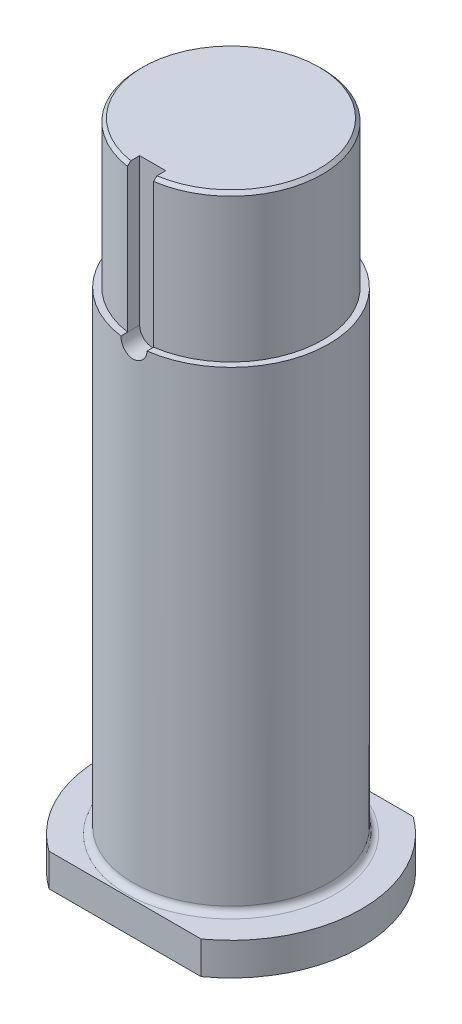
from build123d import *

# Parameters (mm, degrees)
SKETCH2_OUTSIDE_W   = 127.956
SKETCH2_OUTSIDE_H   = 127.956
SKETCH2_OUTSIDE_W_2 = 130
SKETCH2_OUTSIDE_H_2 = 65
CUT_EXTRUDE1_DEPTH  = 10
CUT_EXTRUDE2_REACH  = 213.642
CHAMFER1_SIZE       = 1
FILLET2_R           = 2


with BuildPart() as part:
    # Sketch1 → Revolve1 (revolve)
    with BuildSketch(Plane.XY, mode=Mode.PRIVATE) as revolve1_sk:
        Polygon((0, 0), (40, 0), (40, 10), (30, 10), (30, 155), (28, 155), (28, 200), (0, 200), align=None)
    revolve(revolve1_sk.sketch.rotate(Axis((0, 0, 0), (0, -1, 0)), 90), axis=Axis((0, 0, 0), (0, -1, 0)))

    # Sketch2 outside → Cut-Extrude1 (cut)
    with BuildSketch(Plane(origin=(0, 0, 0), x_dir=(1, 0, 0), z_dir=(0, 1, 0))):
        Rectangle(SKETCH2_OUTSIDE_W, SKETCH2_OUTSIDE_H)
        Rectangle(SKETCH2_OUTSIDE_W_2, SKETCH2_OUTSIDE_H_2, mode=Mode.SUBTRACT)
    extrude(amount=CUT_EXTRUDE1_DEPTH, mode=Mode.SUBTRACT)

    # Sketch3 → Cut-Extrude2 (cut, up to next)
    with BuildSketch(Plane.XY.offset(24), mode=Mode.PRIVATE) as cut_extrude2_sk1:
        with BuildLine():
            Line((4, 200), (4, 155))
            ThreePointArc((4, 155), (0, 151), (-4, 155))
            Line((-4, 155), (-4, 200))
            ThreePointArc((-4, 200), (0, 204), (4, 200))
        make_face()
    cut_extrude2_tool1 = extrude(cut_extrude2_sk1.sketch, amount=CUT_EXTRUDE2_REACH, mode=Mode.PRIVATE) & part.part
    add(cut_extrude2_tool1.solids().sort_by_distance((0, 177.5, 24))[0], mode=Mode.SUBTRACT)

    # Chamfer1
    chamfer1_edges = [part.edges().sort_by_distance(p)[0] for p in [
        (0, 200, -28),
    ]]
    chamfer(chamfer1_edges, length=CHAMFER1_SIZE)

    # Fillet2
    fillet2_edges = [part.edges().sort_by_distance(p)[0] for p in [
        (0, 10, -30),
    ]]
    fillet(fillet2_edges, radius=FILLET2_R)


solid = part.part
